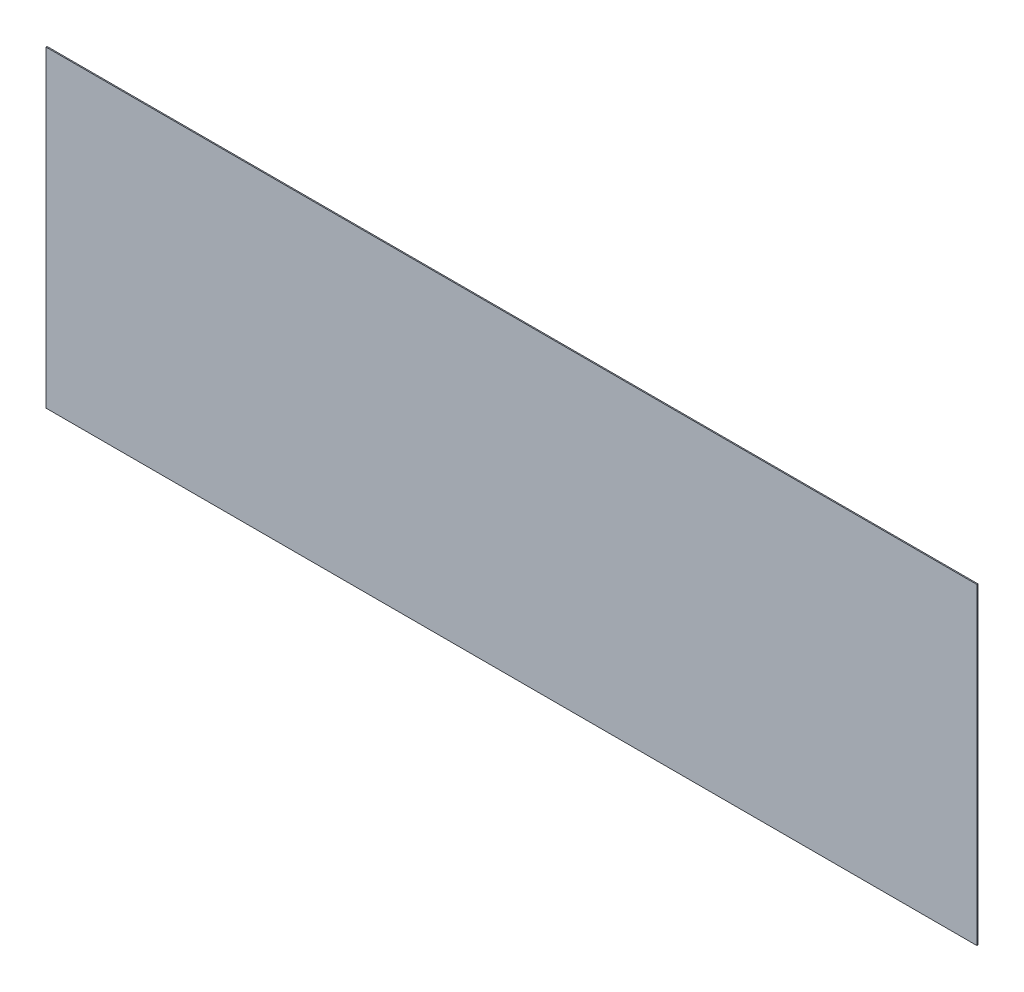
from build123d import *

# Parameters (mm, degrees)
SKETCH1_W           = 1280
SKETCH1_H           = 430
BOSS_EXTRUDE1_DEPTH = 1.5


with BuildPart() as part:
    # Sketch1 → Boss-Extrude1 (new body)
    with BuildSketch(Plane.XY):
        with Locations((640, 215)):
            Rectangle(SKETCH1_W, SKETCH1_H)
    extrude(amount=BOSS_EXTRUDE1_DEPTH)


solid = part.part
